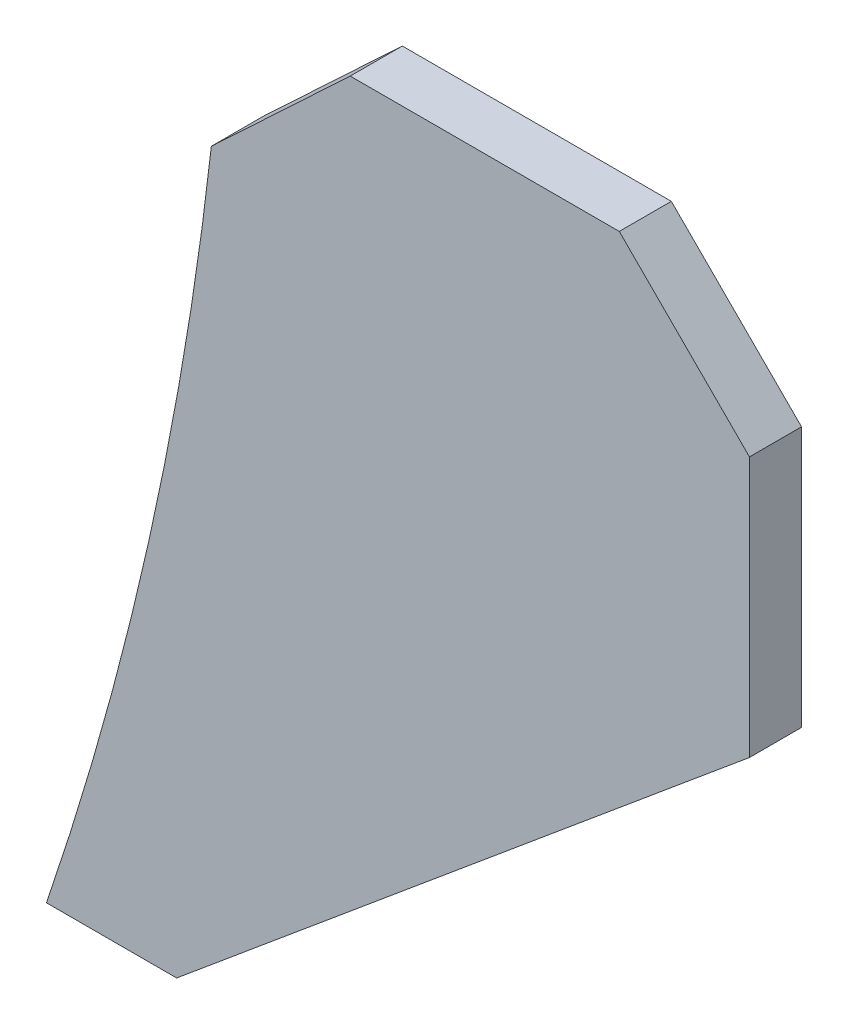
from build123d import *

# Parameters (mm, degrees)
BOSS_EXTRUDE1_DEPTH = 6


with BuildPart() as part:
    # Sketch1 → Boss-Extrude1 (new body)
    with BuildSketch(Plane.XY):
        with BuildLine():
            Line((0, 0), (15, 0))
            Line((15, 0), (81, 55))
            Line((81, 55), (81, 85))
            Line((81, 85), (66, 100))
            Line((66, 100), (35, 100))
            Line((35, 100), (19, 85))
            ThreePointArc((19, 85), (11.791612432, 41.987757221), (0, 0))
        make_face()
    extrude(amount=BOSS_EXTRUDE1_DEPTH)


solid = part.part
